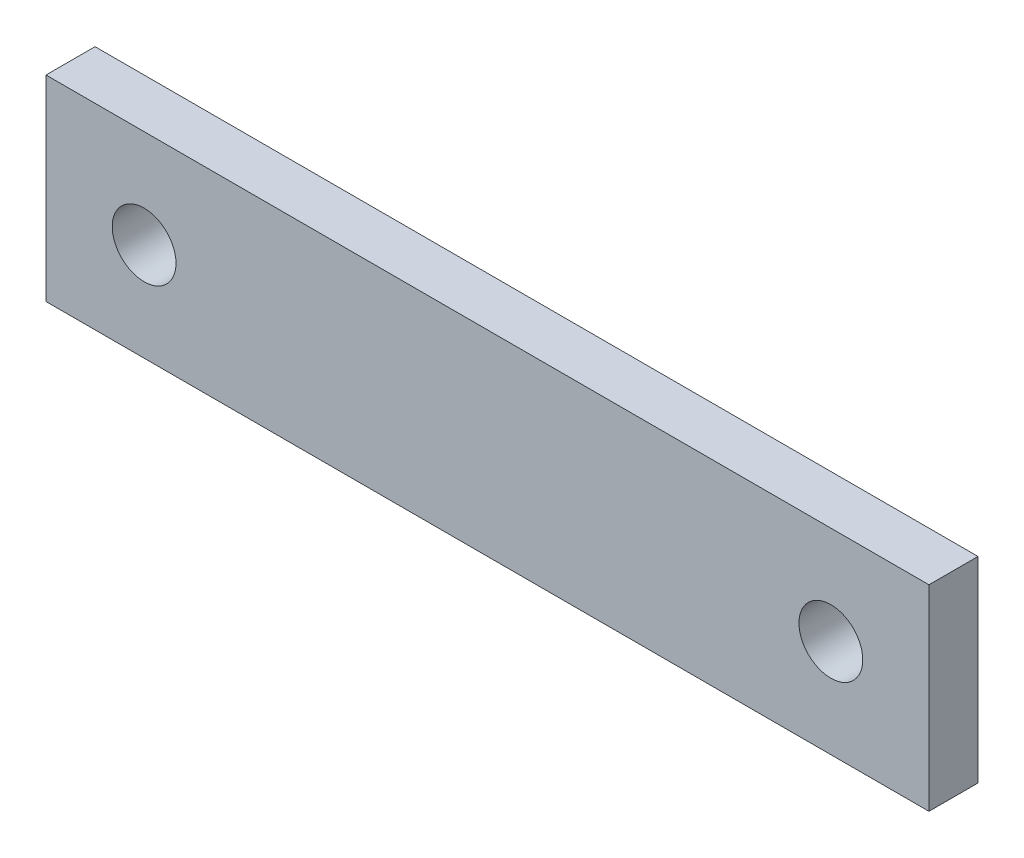
from build123d import *

# Parameters (mm, degrees)
SKETCH1_W                  = 180
SKETCH1_H                  = 40
BOSS_EXTRUDE1_DEPTH        = 5
F_13_0_13_DIAMETER_HOLE1_D = 13


with BuildPart() as part:
    # Sketch1 → Boss-Extrude1 (new, symmetric)
    with BuildSketch(Plane.XY):
        Rectangle(SKETCH1_W, SKETCH1_H)
    extrude(amount=BOSS_EXTRUDE1_DEPTH, both=True)

    # Ø13.0 (13) Diameter Hole1 (through all)
    with Locations(Plane.XY.offset(5)):
        with Locations((-70, 0), (70, 0)):
            Hole(F_13_0_13_DIAMETER_HOLE1_D / 2)


solid = part.part
